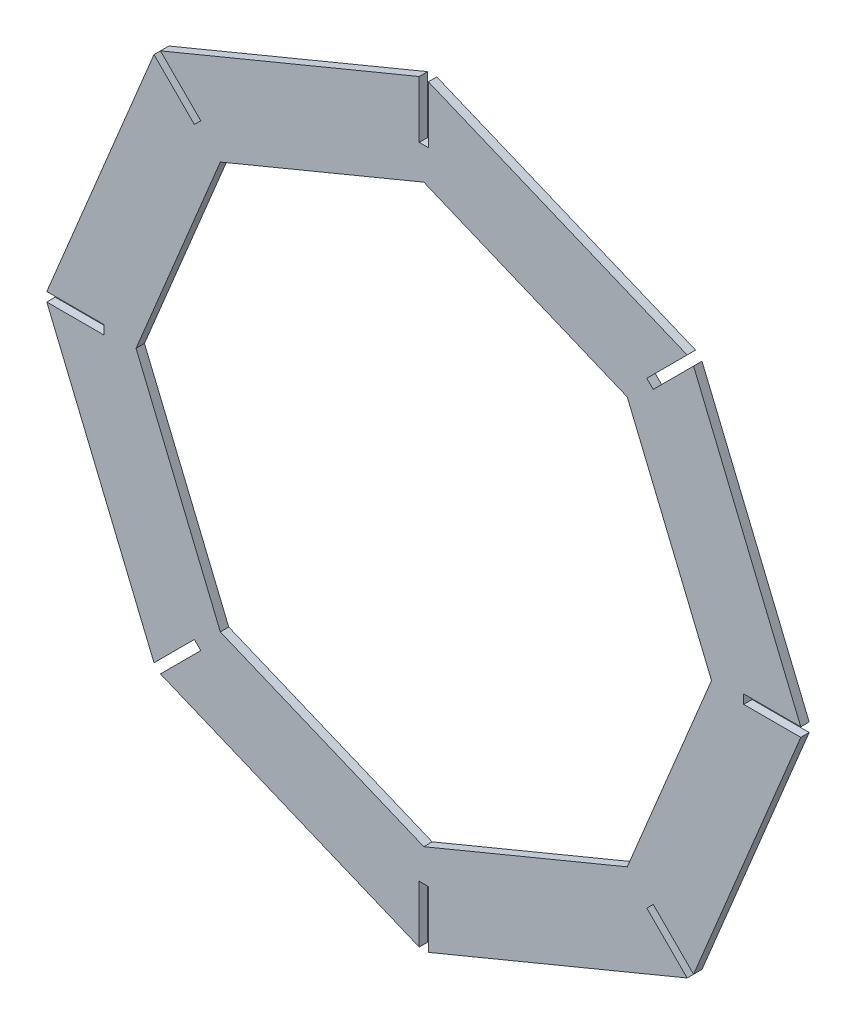
SolidWorks part; units mm, degrees
ref_plane "前视基准面" through (0, 0, 0) normal (0, 0, 1) x (1, 0, 0)
ref_plane "上视基准面" through (0, 0, 0) normal (0, 1, 0) x (1, 0, 0)
ref_plane "右视基准面" through (0, 0, 0) normal (1, 0, 0) x (0, 0, -1)
sketch "草图1" plane through (0, 0, 0) normal (0, 0, 1) x (1, 0, 0)
  line L0 (159.099, 159.099) -> (0, 225)
  line L1 (-159.099, 159.099) -> (-225, 0)
  line L2 (-225, 0) -> (-159.099, -159.099)
  line L3 (-159.099, -159.099) -> (0, -225)
  line L4 (0, -225) -> (159.099, -159.099)
  line L5 (159.099, -159.099) -> (225, 0)
  line L6 (225, 0) -> (159.099, 159.099)
  line L7 (0, 225) -> (-159.099, 159.099)
  line L8 (0, 225) -> (0, 0) construction
  circle A0 centre (0, 0) radius 207.8729 construction
  dimension "D1" = 450
extrude "凸台-拉伸1" add sketch "草图1" along normal blind 5
sketch "草图2" plane through (0, 0, 5) normal (0, 0, 1) x (1, 0, 0)
  line L8 (0, 170.8804) -> (-120.8307, 120.8307)
  line L9 (0, 170.8804) -> (-120.8307, 120.8307)
  line L10 (-120.8307, 120.8307) -> (-170.8804, 0)
  line L11 (-120.8307, 120.8307) -> (-170.8804, 0)
  line L12 (-170.8804, 0) -> (-120.8307, -120.8307)
  line L13 (-170.8804, 0) -> (-120.8307, -120.8307)
  line L14 (-120.8307, -120.8307) -> (0, -170.8804)
  line L15 (-120.8307, -120.8307) -> (0, -170.8804)
  line L16 (0, -170.8804) -> (120.8307, -120.8307)
  line L17 (0, -170.8804) -> (120.8307, -120.8307)
  line L24 (120.8307, -120.8307) -> (170.8804, 0)
  line L25 (120.8307, -120.8307) -> (170.8804, 0)
  line L26 (170.8804, 0) -> (120.8307, 120.8307)
  line L27 (170.8804, 0) -> (120.8307, 120.8307)
  line L28 (120.8307, 120.8307) -> (0, 170.8804)
  line L29 (120.8307, 120.8307) -> (0, 170.8804)
  dimension "D1" = 50
extrude "切除-拉伸1" cut sketch "草图2" against normal blind 606
sketch "草图3" plane through (0, 0, 5) normal (0, 0, 1) x (1, 0, 0)
  circle A0 centre (0, 0) radius 36.8451
sketch "草图4" plane through (0, 0, 5) normal (0, 0, 1) x (1, 0, 0)
  line L0 (185.757, -181.9386) -> (136.2595, -132.4411)
  line L1 (260, -2.7) -> (190, -2.7)
  line L2 (260, -2.7) -> (260, 2.7)
  line L3 (260, 2.7) -> (190, 2.7)
  line L4 (190, -2.7) -> (190, 2.7)
  line L5 (260, -2.7) -> (190, 2.7) construction
  line L6 (260, 2.7) -> (190, -2.7) construction
  line L7 (132.4411, -136.2595) -> (136.2595, -132.4411)
  line L8 (181.9386, -185.757) -> (132.4411, -136.2595)
  line L9 (181.9386, -185.757) -> (185.757, -181.9386)
  line L10 (2.7, -260) -> (2.7, -190)
  line L11 (-2.7, -190) -> (2.7, -190)
  line L12 (-2.7, -260) -> (-2.7, -190)
  line L13 (-2.7, -260) -> (2.7, -260)
  line L14 (-181.9386, -185.757) -> (-132.4411, -136.2595)
  line L15 (-136.2595, -132.4411) -> (-132.4411, -136.2595)
  line L16 (-185.757, -181.9386) -> (-136.2595, -132.4411)
  line L17 (-185.757, -181.9386) -> (-181.9386, -185.757)
  line L18 (-260, -2.7) -> (-190, -2.7)
  line L19 (-190, 2.7) -> (-190, -2.7)
  line L20 (-260, 2.7) -> (-190, 2.7)
  line L21 (-260, 2.7) -> (-260, -2.7)
  line L22 (-185.757, 181.9386) -> (-136.2595, 132.4411)
  line L23 (-132.4411, 136.2595) -> (-136.2595, 132.4411)
  line L24 (-181.9386, 185.757) -> (-132.4411, 136.2595)
  line L25 (-181.9386, 185.757) -> (-185.757, 181.9386)
  line L26 (-2.7, 260) -> (-2.7, 190)
  line L27 (2.7, 190) -> (-2.7, 190)
  line L28 (2.7, 260) -> (2.7, 190)
  line L29 (2.7, 260) -> (-2.7, 260)
  line L30 (181.9386, 185.757) -> (132.4411, 136.2595)
  line L31 (136.2595, 132.4411) -> (132.4411, 136.2595)
  line L32 (185.757, 181.9386) -> (136.2595, 132.4411)
  line L33 (185.757, 181.9386) -> (181.9386, 185.757)
  point P0 (225, 0)
  point P37 (0, 0)
  dimension "D1" = 5.4
  dimension "D2" = 70
  dimension "D3" = 8
extrude "切除-拉伸2" cut sketch "草图4" against normal blind 10
